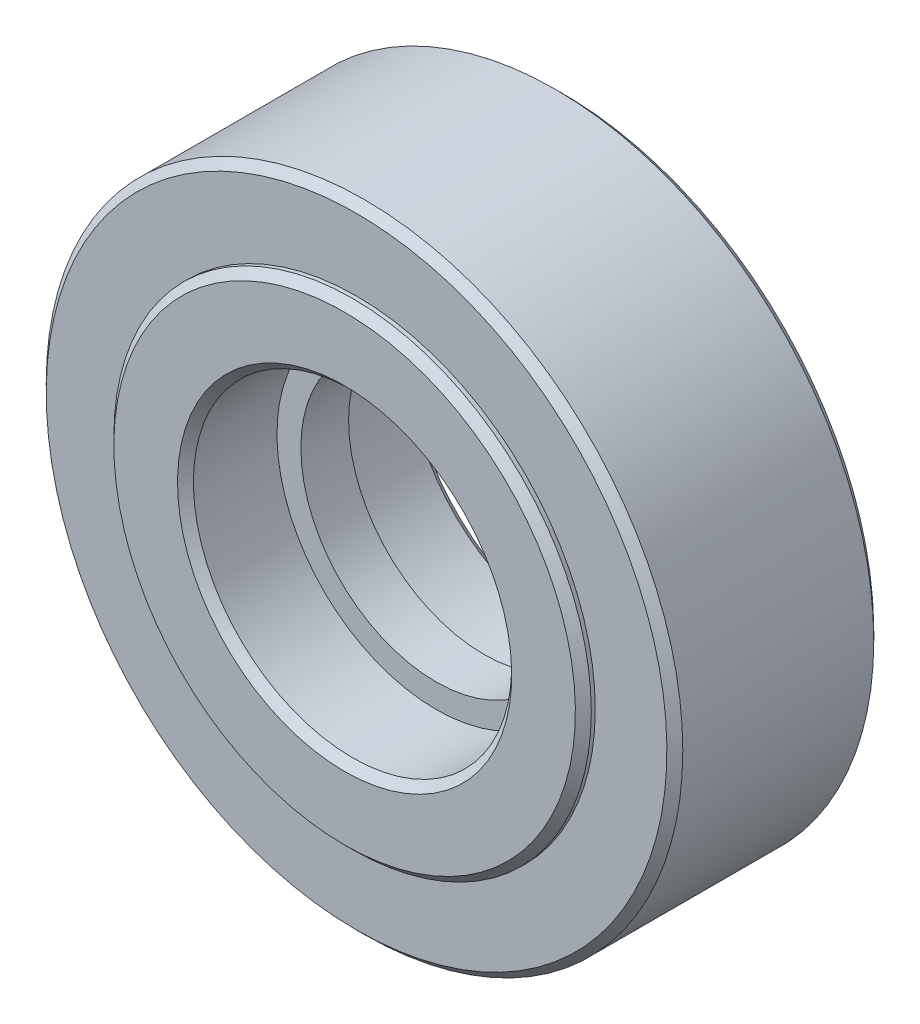
from build123d import *

# Parameters (mm, degrees)
SKETCH_1_3_2_W = 1.5
SKETCH_1_3_2_H = 10
CHAMFER1_SIZE  = 1
CHAMFER2_SIZE  = 1


with BuildPart() as part:
    # Sketch 1_3 → Revolve1 (revolve)
    with BuildSketch(Plane(origin=(0, 0, 0), x_dir=(0, 0, -1), z_dir=(1, 0, 0)), mode=Mode.PRIVATE) as revolve1_sk:
        Polygon((-13, 40), (-13, 30), (-9.5, 30), (-9.5, 27), (-3.5, 27), (-3.5, 30), (3.5, 30), (3.5, 27), (9.5, 27), (9.5, 30), (13, 30), (13, 40), align=None)
    revolve(revolve1_sk.sketch.rotate(Axis((0, 0, 13), (0, 0, -1)), 180), axis=Axis((0, 0, 13), (0, 0, -1)))

    # Chamfer1
    chamfer1_edges = [part.edges().sort_by_distance(p)[0] for p in [
        (0, 40, 13),
        (0, 40, -13),
    ]]
    chamfer(chamfer1_edges, length=CHAMFER1_SIZE)


with BuildPart() as body_2:
    # Sketch 1_3 2 → Revolve2 (revolve)
    with BuildSketch(Plane(origin=(0, 0, 0), x_dir=(0, 0, -1), z_dir=(1, 0, 0)), mode=Mode.PRIVATE) as revolve2_sk:
        Polygon((-13, 30), (-13, 20), (-3, 20), (-3, 17), (3, 17), (3, 20), (13, 20), (13, 30), (9.5, 30), (9.5, 27), (3.5, 27), (3.5, 30), (-3.5, 30), (-3.5, 27), (-9.5, 27), (-9.5, 30), align=None)
        with Locations((-13.75, 25)):
            Rectangle(SKETCH_1_3_2_W, SKETCH_1_3_2_H)
        with Locations((13.75, 25)):
            Rectangle(SKETCH_1_3_2_W, SKETCH_1_3_2_H)
    revolve(revolve2_sk.sketch.rotate(Axis((0, 0, 13), (0, 0, -1)), 180), axis=Axis((0, 0, 13), (0, 0, -1)))

    # Chamfer2
    chamfer2_edges = [body_2.edges().sort_by_distance(p)[0] for p in [
        (0, 30, -14.5),
        (0, 20, -14.5),
        (0, 20, 14.5),
        (0, 30, 14.5),
    ]]
    chamfer(chamfer2_edges, length=CHAMFER2_SIZE)


solid = Compound([part.part, body_2.part])
